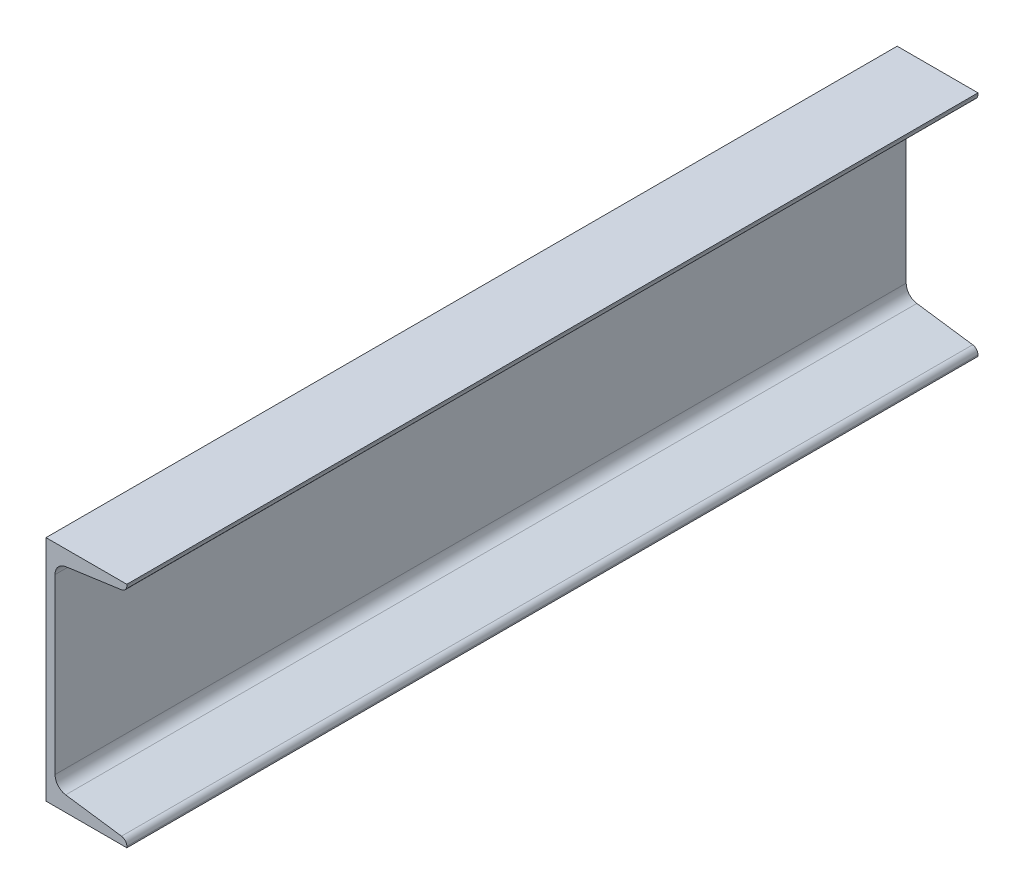
from build123d import *

# Parameters (mm, degrees)
EXTRUDE_1_DEPTH = 895


with BuildPart() as part:
    # 草图1 → 凸台-拉伸1 (new body)
    with BuildSketch(Plane.XY):
        with BuildLine():
            Line((0, 0), (-85, 0))
            Line((-85, 0), (-85, -240))
            Line((-85, -240), (0, -240))
            Line((0, -240), (0, -238.623349271))
            ThreePointArc((0, -238.623349271), (-1.594387729, -234.358965582), (-5.595374844, -232.186606824))
            Line((-5.595374844, -232.186606824), (-64.309250312, -223.934909757))
            ThreePointArc((-64.309250312, -223.934909757), (-72.311224543, -219.59019224), (-75.5, -211.061424863))
            Line((-75.5, -211.061424863), (-75.5, -28.938575137))
            ThreePointArc((-75.5, -28.938575137), (-72.311224543, -20.40980776), (-64.309250312, -16.065090243))
            Line((-64.309250312, -16.065090243), (-5.595374844, -7.813393176))
            ThreePointArc((-5.595374844, -7.813393176), (-1.594387729, -5.641034418), (0, -1.376650729))
            Line((0, -1.376650729), (0, 0))
        make_face()
    extrude(amount=EXTRUDE_1_DEPTH)


solid = part.part
